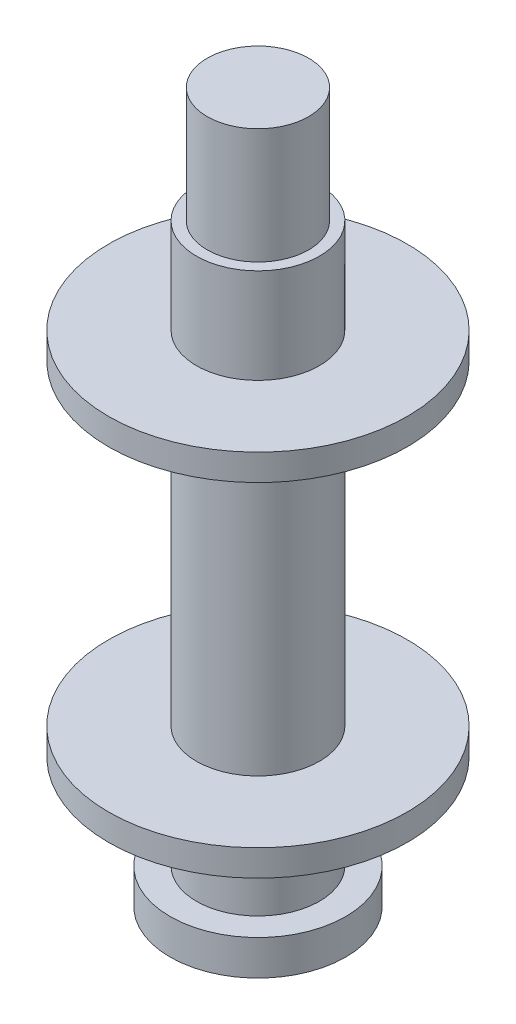
from build123d import *

# Parameters (mm, degrees)
SKETCH1_R           = 5
BOSS_EXTRUDE1_DEPTH = 2
SKETCH2_R           = 3.5
BOSS_EXTRUDE2_DEPTH = 5.4
SKETCH3_R           = 8.5
BOSS_EXTRUDE3_DEPTH = 1.5
SKETCH4_R           = 3.5
BOSS_EXTRUDE4_DEPTH = 18
SKETCH5_R           = 8.5
BOSS_EXTRUDE5_DEPTH = 1.5
SKETCH6_R           = 3.5
BOSS_EXTRUDE6_DEPTH = 5.4
SKETCH7_R           = 2.885
BOSS_EXTRUDE7_DEPTH = 6.57


with BuildPart() as part:
    # Sketch1 → Boss-Extrude1 (new body)
    with BuildSketch(Plane(origin=(0, 0, 0), x_dir=(1, 0, 0), z_dir=(0, 1, 0))):
        with Locations(Location((0, 0, 0), (0, 0, 270))):
            Circle(SKETCH1_R)
    extrude(amount=BOSS_EXTRUDE1_DEPTH)

    # Sketch2 → Boss-Extrude2 (add)
    with BuildSketch(Plane(origin=(0, 2, 0), x_dir=(1, 0, 0), z_dir=(0, 1, 0))):
        with Locations(Location((0, 0, 0), (0, 0, 90))):
            Circle(SKETCH2_R)
    extrude(amount=BOSS_EXTRUDE2_DEPTH)

    # Sketch3 → Boss-Extrude3 (add)
    with BuildSketch(Plane(origin=(0, 7.4, 0), x_dir=(1, 0, 0), z_dir=(0, 1, 0))):
        with Locations(Location((0, 0, 0), (0, 0, 270))):
            Circle(SKETCH3_R)
    extrude(amount=BOSS_EXTRUDE3_DEPTH)

    # Sketch4 → Boss-Extrude4 (add)
    with BuildSketch(Plane(origin=(0, 8.9, 0), x_dir=(1, 0, 0), z_dir=(0, 1, 0))):
        with Locations(Location((0, 0, 0), (0, 0, 90))):
            Circle(SKETCH4_R)
    extrude(amount=BOSS_EXTRUDE4_DEPTH)

    # Sketch5 → Boss-Extrude5 (add)
    with BuildSketch(Plane(origin=(0, 26.9, 0), x_dir=(1, 0, 0), z_dir=(0, 1, 0))):
        with Locations(Location((0, 0, 0), (0, 0, 270))):
            Circle(SKETCH5_R)
    extrude(amount=BOSS_EXTRUDE5_DEPTH)

    # Sketch6 → Boss-Extrude6 (add)
    with BuildSketch(Plane(origin=(0, 28.4, 0), x_dir=(1, 0, 0), z_dir=(0, 1, 0))):
        with Locations(Location((0, 0, 0), (0, 0, 90))):
            Circle(SKETCH6_R)
    extrude(amount=BOSS_EXTRUDE6_DEPTH)

    # Sketch7 → Boss-Extrude7 (add)
    with BuildSketch(Plane(origin=(0, 33.8, 0), x_dir=(1, 0, 0), z_dir=(0, 1, 0))):
        with Locations(Location((0, 0, 0), (0, 0, 270))):
            Circle(SKETCH7_R)
    extrude(amount=BOSS_EXTRUDE7_DEPTH)


solid = part.part
